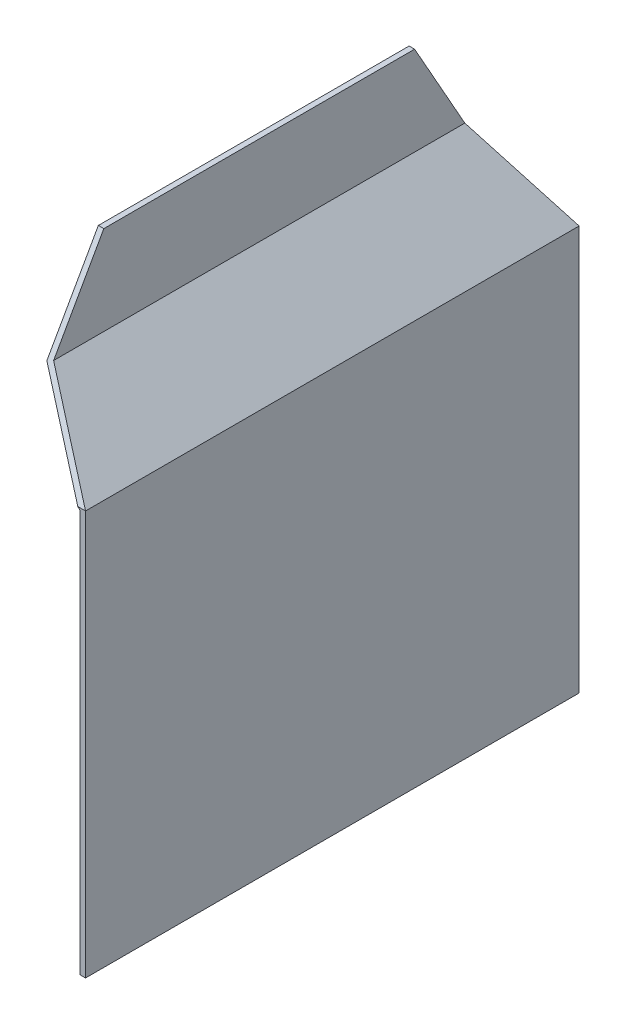
SolidWorks part; units mm, degrees
ref_plane "前视基准面" through (0, 0, 0) normal (0, 0, 1) x (1, 0, 0)
ref_plane "上视基准面" through (0, 0, 0) normal (0, 1, 0) x (1, 0, 0)
ref_plane "右视基准面" through (0, 0, 0) normal (1, 0, 0) x (0, 0, -1)
sketch "草图1" plane through (0, 0, 0) normal (0, 0, 1) x (1, 0, 0)
  line L0 (0, 0) -> (0, -50)
  line L1 (3, 0) -> (3, -48.7574)
  line L2 (43, -88.7574) -> (3, -48.7574)
  line L3 (43, -88.7574) -> (43, -310)
  line L4 (0, 0) -> (3, 0)
  line L5 (40, -90) -> (0, -50)
  line L6 (40, -90) -> (40, -310)
  line L7 (40, -310) -> (43, -310)
  dimension "D1" = 3
extrude "凸台-拉伸1" add sketch "草图1" along normal blind 270
sketch "草图2" plane through (43, 0, 0) normal (1, 0, 0) x (0, 0, -1)
  line L0 (-270, 0) -> (-220, 0)
  line L1 (-220, 0) -> (-270, -88.7574)
  line L2 (-270, 0) -> (0, 0) construction
  line L3 (-270, -88.7574) -> (-270, 0)
  line L4 (0, 0) -> (-50, 0)
  line L5 (-50, 0) -> (0, -88.7574)
  line L6 (0, -88.7574) -> (0, 0)
extrude "切除-拉伸2" cut sketch "草图2" against normal blind 270
